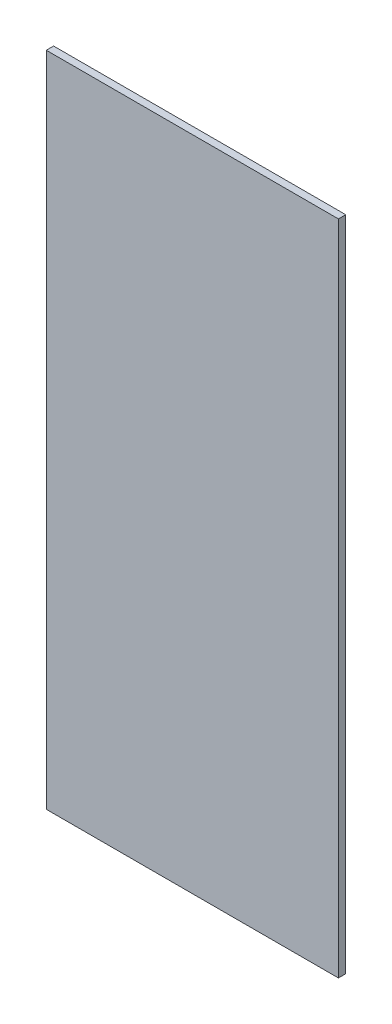
SolidWorks part; units mm, degrees
ref_plane "前视基准面" through (0, 0, 0) normal (0, 0, 1) x (1, 0, 0)
ref_plane "上视基准面" through (0, 0, 0) normal (0, 1, 0) x (1, 0, 0)
ref_plane "右视基准面" through (0, 0, 0) normal (1, 0, 0) x (0, 0, -1)
other "Configuration Table"
sketch "草图1" plane through (0, 0, 0) normal (0, 0, 1) x (1, 0, 0)
  line L1 (-400, -900) -> (400, -900)
  line L2 (-400, -900) -> (-400, 900)
  line L3 (-400, 900) -> (400, 900)
  line L4 (400, -900) -> (400, 900)
  line L5 (-400, -900) -> (400, 900) construction
  line L6 (-400, 900) -> (400, -900) construction
  point P0 (0, 0)
  dimension "D1" = 1800
  dimension "D2" = 800
extrude "凸台-拉伸1" add sketch "草图1" along normal blind 20
